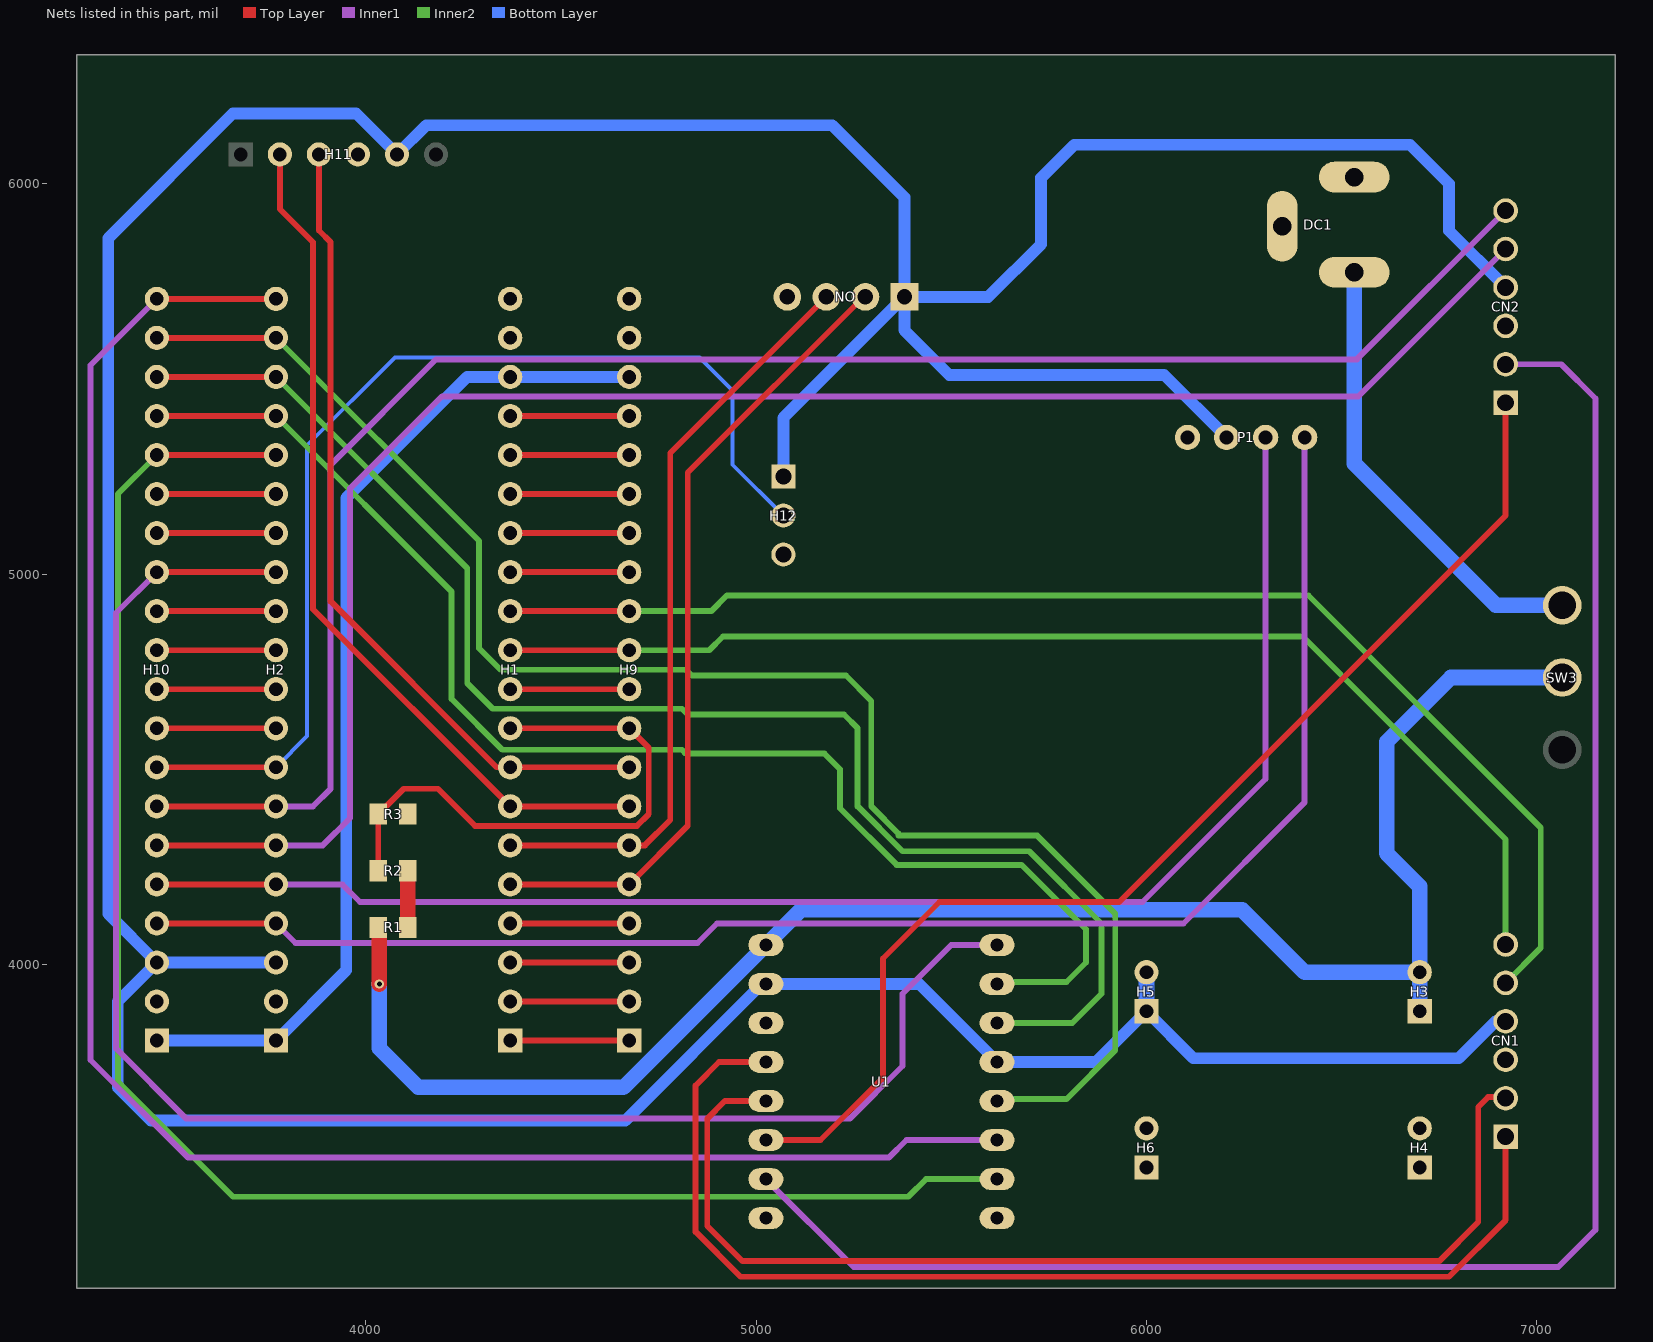
[diagram p0: the nets of this part, all layers, seen from the top]
# Altium PCB MISC51780.pcbdoc (part 2 of 2)
Units mil, origin at the board's own origin, x right, y up, seen from the top; angles counter-clockwise.
Board outline 3940.5 x 3159.99 mil, 4 copper layers (Top Layer, Inner1, Inner2, Bottom Layer), stack 62.206 mil thick; 24 components, 44 nets, 145 pads, 1 vias.

## Via types
v1: diameter 24, hole 12, Top Layer to Bottom Layer, 1 vias

## Nets (pads, with @x,y where several pads share a name; then routed paths per layer and width w, separated by ;. In a path a pad name is that pad's centre, name@x,y a point inside that pad or via, vN(x,y) a via of type N, cw(c..) or ccw(c..) an arc to the next point about the centre after c; other vN are vias at no path point)
3.3V: H1.18 H2.1 H9.18 H10.1 | length 2623
  Bottom Layer w30: H10.1@3465,3805 H2.1@3770,3805 3950,3985 3950,5195 4260,5505 H1.18@4370,5505 H9.18@4675,5505
5V: CN1.4 CN2.4 H2.3 H5.1 H5.2 H10.3 H11.5 H12.1 NO.1 P1.2 U1.2 U1.13 | length 12848.4
  Bottom Layer w30: H2.3@3770,4005 H10.3@3465,4005 ; H12.1@5070,5250 5070,5400 NO.1@5380,5710 ; P1.2@6205.1,5350 6045.1,5510 5495,5510 5380,5625 NO.1@5380,5710 ; CN1.4@6920,3854.21 6894.2,3854.2 6800,3760 6120,3760 H5.1@6000,3880 5870,3750 5617.3,3750 5417.3,3950 U1.2@5025,3950 5015,3950 4665,3600 3450,3600 3365,3685 3365,3905 H10.3@3465,4005 ; CN2.4@6920,5734.21 6775,5879.2 6775,6000 6675,6100 5815,6100 5730,6015 5730,5845 5595,5710 NO.1@5380,5710 ; H10.3@3465,4005 3340,4130 3340,5860 3660,6180 3975,6180 H11.5@4080,6075 4155,6150 5195,6150 5380,5965 NO.1@5380,5710
  Bottom Layer w40: H5.1@6000,3880 H5.2@6000,3980
$1N34: DC1.1 SW3.1 | length 1173.2
  Bottom Layer w40: DC1.1@6532.52,5772.96 6532.5,5282.5 6895,4920 SW3.1@7065,4920.04
$1N113: R1.1 R2.2 | length 145
  Top Layer w40: R1.1@4108.04,4095 R2.2@4108.04,4240
ADC: H1.9 H9.9 R2.1 R3.2 | length 1462.4
  Top Layer w15: R2.1@4031.96,4240 R3.2@4031.96,4385 4097,4450 4185,4450 4280,4355 4695,4355 4725,4385 4725,4555 H9.9@4675,4605 H1.9@4370,4605
AIN1: H2.18 H10.18 U1.14 | length 3768.6
  Top Layer w15: H10.18@3465,5505 H2.18@3770,5505
  Inner2 w15: H2.18@3770,5505 4260,5015 4260,4720 4325,4655 4810,4655 4825,4640 5225,4640 5260,4605 5260,4405 5375,4290 5700,4290 5885,4105 5885,3925 5810,3850 U1.14@5617.3,3850
AIN2: H2.17 H10.17 U1.15 | length 3479.8
  Top Layer w15: H10.17@3465,5405 H2.17@3770,5405
  Inner2 w15: H2.17@3770,5405 4220,4955 4220,4680 4350,4550 4810,4550 4820,4540 5175,4540 5215,4500 5215,4400 5360,4255 5680,4255 5845,4090 5845,4005 5795,3955 5622.3,3955 U1.15@5617.3,3950
AO1: CN1.1 U1.4 | length 2976.4
  Top Layer w15: U1.4@5025,3750 4905,3750 4845,3690 4845,3315 4960,3200 6775,3200 6920,3345 CN1.1@6920.01,3558.93
AO2: CN1.2 U1.5 | length 2873.8
  Top Layer w15: U1.5@5025,3650 4920,3650 4875,3605 4875,3330 4965,3240 6750,3240 6850,3340 6850,3635 6875,3660 6917.4,3660 CN1.2@6920,3657.36
BIN1: H2.19 H10.19 U1.12 | length 4094.7
  Top Layer w15: H10.19@3465,5605 H2.19@3770,5605
  Inner2 w15: H2.19@3770,5605 4290,5085 4290,4810 4345,4755 4820,4755 4835,4740 5230,4740 5295,4675 5295,4405 5365,4335 5365,4330 5720,4330 5920,4130 5920,3780 5795,3655 5622.3,3655 U1.12@5617.3,3650
BIN2: H2.20 H10.20 U1.11 | length 4769.9
  Top Layer w15: H10.20@3465,5705 H2.20@3770,5705
  Inner1 w15: H10.20@3465,5705 3295,5535 3295,3755 3545,3505 5340,3505 5385,3550 U1.11@5617.3,3550
BO1: CN2.2 U1.7 | length 4653.8
  Inner1 w15: U1.7@5025,3450 5250,3225 7055,3225 7150,3320 7150,5450 7062.6,5537.4 CN2.2@6920,5537.36
BO2: CN2.1 U1.6 | length 3025.3
  Top Layer w15: U1.6@5025,3550 5165,3550 5325,3710 5325,4015 5470,4160 5930,4160 6920,5150 CN2.1@6920.01,5438.93
BUZZER: H2.8 H10.8 H12.2 | length 2755.4
  Top Layer w15: H10.8@3465,4505 H2.8@3770,4505
  Bottom Layer w10: H2.8@3770,4505 3850,4585 3850,5330 4075,5555 4855,5555 4940,5470 4940,5280 H12.2@5070,5150
GND: CN1.3 CN2.3 DC1.2 DC1.3 H1.19 H1.20 H2.2 H4.1 H4.2 H6.1 H6.2 H9.19 H9.20 H10.2 H11.4 H12.3 NO.4 P1.1 R3.1 U1.3 U1.8 U1.9
M1A: CN1.6 H1.11 H9.11 | length 3048.8
  Top Layer w15: H1.11@4370,4805 H9.11@4675,4805
  Inner2 w15: H9.11@4675,4805 4880,4805 4915,4840 6400,4840 6920,4320 CN1.6@6920,4051.06
M1B: CN1.5 H1.12 H9.12 | length 3337.7
  Top Layer w15: H1.12@4370,4905 H9.12@4675,4905
  Inner2 w15: H9.12@4675,4905 4885,4905 4925,4945 6415,4945 7010,4350 7010,4042.63 CN1.5@6920.01,3952.63
M2A: CN2.6 H2.7 H10.7 | length 4573.3
  Top Layer w15: H10.7@3465,4405 H2.7@3770,4405
  Inner1 w15: H2.7@3770,4405 3865,4405 3910,4450 3910,5280 4180,5550 6538.9,5550 CN2.6@6920,5931.06
M2B: CN2.5 H2.6 H10.6 | length 4582.7
  Top Layer w15: H10.6@3465,4305 H2.6@3770,4305
  Inner1 w15: H2.6@3770,4305 3890,4305 3960,4375 3960,5220 4195,5455 6542.4,5455 CN2.5@6920.01,5832.63
NRST: H1.17 H9.17 | length 305
  Top Layer w15: H1.17@4370,5405 H9.17@4675,5405
OLED_SCL: H2.5 H10.5 P1.3 | length 3864.1
  Top Layer w15: H10.5@3465,4205 H2.5@3770,4205
  Inner1 w15: H2.5@3770,4205 3940,4205 3985,4160 5990,4160 6305,4475 P1.3@6305.1,5350
OLED_SDA: H2.4 H10.4 P1.4 | length 4044.9
  Top Layer w15: H10.4@3465,4105 H2.4@3770,4105
  Inner1 w15: H2.4@3770,4105 3820,4055 4850,4055 4900,4105 6095,4105 6405.1,4415.1 P1.4@6405.1,5350
PA0: H1.5 H9.5 NO.2 | length 2063.5
  Top Layer w15: H1.5@4370,4205 H9.5@4675,4205 4825,4355 4825,5260 5275,5710 NO.2@5280,5710
PA1: H1.6 H9.6 NO.3 | length 1942.6
  Top Layer w15: H1.6@4370,4305 H9.6@4675,4305 4715,4305 4780,4370 4780,5310 NO.3@5180,5710
PA2: H1.7 H9.7 H11.2 | length 2219.4
  Top Layer w15: H11.2@3780,6075 3780,5935 3865,5850 3865,4910 H1.7@4370,4405 H9.7@4675,4405
PA3: H1.8 H9.8 H11.3 | length 2098.5
  Top Layer w15: H11.3@3880,6075 3880,5880 3910,5850 3910,4930 4335,4505 H1.8@4370,4505 H9.8@4675,4505
PA5: H1.10 H9.10 | length 305
  Top Layer w15: H1.10@4370,4705 H9.10@4675,4705
PA8: H2.16 H10.16 U1.10 | length 4344.6
  Top Layer w15: H10.16@3465,5305 H2.16@3770,5305
  Inner2 w15: H10.16@3465,5305 3365,5205 3365,3700 3660,3405 5390,3405 5435,3450 U1.10@5617.3,3450
PA9: H2.15 H10.15 | length 305
  Top Layer w15: H10.15@3465,5205 H2.15@3770,5205
PA10: H2.14 H10.14 | length 305
  Top Layer w15: H10.14@3465,5105 H2.14@3770,5105
PA11: H2.13 H10.13 U1.16 | length 4193
  Top Layer w15: H10.13@3465,5005 H2.13@3770,5005
  Inner1 w15: H10.13@3465,5005 3360,4900 3360,3785 3540,3605 5240,3605 5375,3740 5375,3925 5500,4050 U1.16@5617.3,4050
PA12: H2.12 H10.12 | length 305
  Top Layer w15: H10.12@3465,4905 H2.12@3770,4905
PA15: H2.11 H10.11 | length 305
  Top Layer w15: H10.11@3465,4805 H2.11@3770,4805
PB0: H1.13 H9.13 | length 305
  Top Layer w15: H1.13@4370,5005 H9.13@4675,5005
PB1: H1.14 H9.14 | length 305
  Top Layer w15: H1.14@4370,5105 H9.14@4675,5105
PB3: H2.10 H10.10 | length 305
  Top Layer w15: H10.10@3465,4705 H2.10@3770,4705
PB4: H2.9 H10.9 | length 305
  Top Layer w15: H10.9@3465,4605 H2.9@3770,4605
PB10: H1.15 H9.15 | length 305
  Top Layer w15: H1.15@4370,5205 H9.15@4675,5205
PB11: H1.16 H9.16 | length 305
  Top Layer w15: H1.16@4370,5305 H9.16@4675,5305
PC13: H1.2 H9.2 | length 305
  Top Layer w15: H1.2@4370,3905 H9.2@4675,3905
PC14: H1.3 H9.3 | length 305
  Top Layer w15: H1.3@4370,4005 H9.3@4675,4005
PC15: H1.4 H9.4 | length 305
  Top Layer w15: H1.4@4370,4105 H9.4@4675,4105
VBAT: H1.1 H9.1 | length 305
  Top Layer w15: H1.1@4370,3805 H9.1@4675,3805
VBAT_IN: H3.1 H3.2 R1.2 SW3.2 U1.1 | length 4516
  Top Layer w40: R1.2@4031.96,4095 4035,4092 v1(4035,3950)
  Bottom Layer w40: v1(4035,3950) 4035,3785 4135,3685 4660,3685 U1.1@5025,4050 5115,4140 6245,4140 6405,3980 H3.2@6700,3980 ; H3.1@6700,3880 H3.2@6700,3980 ; SW3.2@7065,4735 6780,4735 6615,4570 6615,4285 6700,4200 H3.2@6700,3980
pads on no net: H11.1 H11.6 SW3.3

## Polygon pours and split planes (outlines as drawn)
GND on Bottom Layer (solid, remove dead copper, pour order 2): 3000,6570 3070,6500 7370,6500 7290,6420 7290,3000 7210,3080 3030,3080 3040,3090 3210,3090
GND on Inner1 (solid, remove dead copper): 3135,6455 3175,6415 7325,6415 7285,6375 7285,3005 7235,3055 3105,3055
GND on Inner2 (solid, remove dead copper): 3125,6475 3175,6425 7385,6425 7295,6335 7295,3015 7255,3055 3095,3055 3095,3085
GND on Top Layer (solid, remove dead copper, pour order 0): 3125.03,3045 3135,6435 7315,6435 7285,6405 7285,3055 7275,3045

## Keep-outs
Board Outline Layer:
  region: 5545,4450 cw(c5485,4450) 5425,4450 cw(c5485,4450)
  circle w0.1: c5485,4450 r60
  region: 5545,4450 5544.62,4443.28 5543.5,4436.65 5541.63,4430.18 5539.06,4423.97 5535.8,4418.08 5531.91,4412.59 5527.43,4407.57 5522.41,4403.09 5516.92,4399.2 5511.03,4395.94 5504.82,4393.37 5498.35,4391.5 5491.72,4390.38 5485,4390 5478.28,4390.38 5471.65,4391.5 5465.18,4393.37 5458.97,4395.94 5453.08,4399.2 5447.59,4403.09 5442.57,4407.57 5438.09,4412.59 5434.2,4418.08 5430.94,4423.97 5428.37,4430.18 5426.5,4436.65 5425.38,4443.28 5425,4450 5425.38,4456.72 5426.5,4463.35 5428.37,4469.82 5430.94,4476.03 5434.2,4481.92 5438.09,4487.41 5442.57,4492.43 5447.59,4496.91 5453.08,4500.8 5458.97,4504.06 5465.18,4506.63 5471.65,4508.5 5478.28,4509.62 5485,4510 5491.72,4509.62 5498.35,4508.5 5504.82,4506.63 5511.03,4504.06 5516.92,4500.8 5522.41,4496.91 5527.43,4492.43 5531.91,4487.41 5535.8,4481.92 5539.06,4476.03 5541.63,4469.82 5543.5,4463.35 5544.62,4456.72
  region: 5545,5030 cw(c5485,5030) 5425,5030 cw(c5485,5030)
  circle w0.1: c5485,5030 r60
  region: 5545,5030 5544.62,5023.28 5543.5,5016.65 5541.63,5010.18 5539.06,5003.97 5535.8,4998.08 5531.91,4992.59 5527.43,4987.57 5522.41,4983.09 5516.92,4979.2 5511.03,4975.94 5504.82,4973.37 5498.35,4971.5 5491.72,4970.38 5485,4970 5478.28,4970.38 5471.65,4971.5 5465.18,4973.37 5458.97,4975.94 5453.08,4979.2 5447.59,4983.09 5442.57,4987.57 5438.09,4992.59 5434.2,4998.08 5430.94,5003.97 5428.37,5010.18 5426.5,5016.65 5425.38,5023.28 5425,5030 5425.38,5036.72 5426.5,5043.35 5428.37,5049.82 5430.94,5056.03 5434.2,5061.92 5438.09,5067.41 5442.57,5072.43 5447.59,5076.91 5453.08,5080.8 5458.97,5084.06 5465.18,5086.63 5471.65,5088.5 5478.28,5089.62 5485,5090 5491.72,5089.62 5498.35,5088.5 5504.82,5086.63 5511.03,5084.06 5516.92,5080.8 5522.41,5076.91 5527.43,5072.43 5531.91,5067.41 5535.8,5061.92 5539.06,5056.03 5541.63,5049.82 5543.5,5043.35 5544.62,5036.72
  lines w10: 3260,3170.01 3260,6330 7200.5,6330 7200.5,3170.01 3260,3170.01

## Other copper
Top Layer:
  region net PA1: 5144.64,5712.22 5182.22,5674.64 5151.19,5670.59 5140.59,5681.19
  region net PA0: 5279.62,5674.57 5244.89,5714.8 5238.57,5684.17 5248.39,5672.79
  region net PA3: 3903.25,6054.5 3856.75,6054.5 3872.5,6032.8 3887.5,6032.8
  region net PA2: 3803.25,6054.5 3756.75,6054.5 3772.5,6032.8 3787.5,6032.8
  region net AO2: 6900.66,3682.22 6897.75,3635.07 6876.74,3652.5 6877.66,3667.5
  region net AO1: 6938.75,3527.44 6901.25,3527.44 6912.5,3504.94 6927.5,3504.94
  region net BO2: 5062.61,3531.25 5062.61,3568.75 5085.11,3557.5 5085.11,3542.5
  region net AO2: 4987.41,3631.25 4987.41,3668.75 4964.91,3657.5 4964.91,3642.5
  region net AO1: 4987.41,3731.25 4987.41,3768.75 4964.91,3757.5 4964.91,3742.5
Inner1:
  region net BO1: 5067.62,3439.13 5034.26,3422 5064.9,3399.5 5086.12,3399.5
  region net PA11: 5579.65,4031.25 5579.65,4068.75 5557.15,4057.5 5557.15,4042.5
Inner2:
  region net PA8: 5579.65,3431.25 5579.65,3468.75 5557.15,3457.5 5557.15,3442.5
Bottom Layer:
  region net VBAT_IN: 6679.5,3956.75 6679.5,4003.25 6657.8,4000 6657.8,3960
  region net VBAT_IN: 6723.25,4000.5 6676.75,4000.5 6680,4022.2 6720,4022.2
  region net VBAT_IN: 6723.25,3959.5 6676.75,3959.5 6680,3937.8 6720,3937.8
  region net 5V: 4049.06,6073.06 4081.94,6105.94 4060.76,6115.45 4039.55,6094.24
  region net 5V: 4078.06,6105.94 4110.94,6073.06 4120.45,6094.24 4099.24,6115.45
  region net 5V: 6172.68,5347.97 6207.13,5382.42 6184.44,5391.87 6163.22,5370.66
  region net VBAT_IN: 7032.45,4698.09 7032.45,4771.91 6998,4755 6998,4715
  region net 5V: 6908.42,3824.92 6892.39,3869.36 6874.04,3855.25 6885.29,3824.07
  region net 5V: 5415.43,5674.57 5344.57,5674.57 5365,5629.57 5395,5629.57
  region net 5V: 5415.43,5745.43 5415.43,5674.57 5460.43,5695 5460.43,5725
  region net 5V: 5344.57,5745.43 5415.43,5745.43 5395,5790.43 5365,5790.43
  region net VBAT_IN: 6669,3911 6731,3911 6720,3971 6680,3971
  region net VBAT_IN: 5008.21,4078 5041.81,4078 5108.26,4104.96 5063.91,4117.18
  region net VBAT_IN: 5041.81,4022 5008.21,4022 4941.76,3995.04 4986.11,3982.82
  region net 5V: 5600.45,3778 5634.05,3778 5573.67,3814.8 5535.65,3810.39
  region net 5V: 5634.05,3722 5634.05,3778 5679.05,3765 5679.05,3735
  region net 5V: 5041.81,3922 5008.21,3978 4959.94,3916.16 4987.95,3901.73
  region net 5V: 5041.81,3922 5041.81,3978 5086.81,3965 5086.81,3935

## Silkscreen, mask and mechanical layers (free items; w line width, h text height)
Top Silkscreen Layer:
  drawing of 82 lines, arcs and shapes, not listed
  text "RX" at 3760,5970 h39
  text "TX" at 3845,5970 h39
  text "GND" at 3930,5970 h39
  text "5V" at 4050,5970 h39
  text "PB12" at 3540,5685 h39
  text "GND" at 4490,5685 h39
  text "USB" at 4015.29,5590 h39
  text "GND" at 4490,5590 h39
  text "PB13" at 3540,5585 h39
  text "Echo" at 5125,5555 h39
  text "Trig" at 5270,5555 h39
  text "GND" at 4995,5550 h39
  text "5V" at 5400,5550 h39
  text "PB14" at 3540,5485 h39
  text "3.3V" at 4475,5485 h39
  text "Note direction" at 3900.29,5445 h80
  text "PB15" at 3540,5390 h39
  text "NRST" at 4465,5390 h39
  text "USB up" at 3905.29,5345 h80
  text "PA8" at 3540,5285 h39
  text "PB11" at 4485,5285 h39
  text "5V" at 5145,5235 h39
  text "PA9" at 3540,5190 h39
  text "PB10" at 4475,5190 h39
  text "IO" at 5145.1,5130.5 h39
  text "PA10" at 3540,5085 h39
  text "PB1" at 4505,5085 h39
  text "GND" at 5142.55,5030.5 h39
  text "ON" at 7040,5005 h80
  text "PA11" at 3545,4985 h39
  text "PB0" at 4495,4985 h39
  text "PA12" at 3540,4885 h39
  text "PA7" at 4495,4885 h39
  text "Buzzer module" at 4905,4875 h98.4
  text "PA6" at 4495,4795 h39
  text "PA15" at 3535,4785 h39
  text "0.96'OLED" at 5975,4755 h80
  text "PB3" at 3535,4690 h39
  text "PA5" at 4495,4690 h39
  text "PA4" at 4490,4590 h39
  text "PB4" at 3535,4585 h39
  text "PA3" at 4490,4490 h39
  text "PB5" at 3535,4485 h39
  text "10K" at 4060,4405 h20 r270
  text "PA2" at 4490,4390 h39
  text "OFF" at 7035,4390 h80
  text "PB6" at 3535,4385 h39
  text "PB7" at 3535,4290 h39
  text "PA1" at 4495,4290 h39
  text "20K" at 4060,4270 h20 r270
  text "PB8" at 3535,4190 h39
  text "PA0" at 4490,4185 h39
  text "20K" at 4060,4120 h20 r270
  text "PC15" at 4470,4090 h39
  text "PB9" at 3535,4085 h39
  text "5V" at 5965,4040 h45
  text "12V" at 6650,4040 h45
  text "PC14" at 4470,3990 h39
  text "5V" at 3535,3980 h39
  text "OUT+" at 6065,3980 h30
  text "IN+" at 6570,3980 h30
  text "GND" at 3540,3885 h39
  text "PC13" at 4470,3885 h39
  text "VBAT" at 4455,3790 h39
  text "3.3V" at 3540,3785 h39
  text "Note direction" at 6230,3615 h60
  text "OUT-" at 6065,3445 h30
  text "IN-" at 6565,3445 h30
  text "GND" at 5940,3370 h45
  text "GND" at 6640,3370 h45
Bottom Silkscreen Layer:
  text "7V-15V input" at 6375,6295 h60 r180
Mechanical Layer:
  circle w0.1: c5485,4450 r60
  circle w0.1: c5485,5030 r60